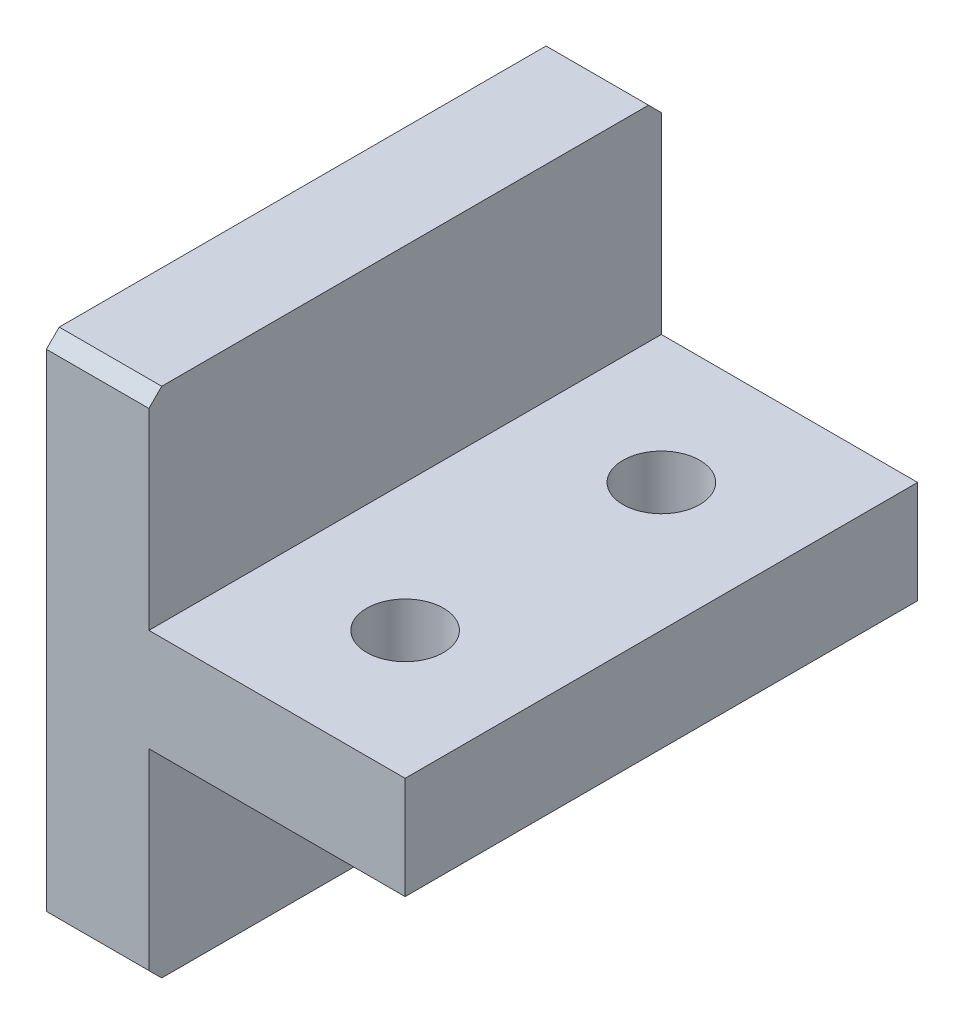
from build123d import *

# Parameters (mm, degrees)
SKETCH1_W               = 8
SKETCH1_H               = 40
BOSS_EXTRUDE1_DEPTH     = 40
CHAMFER1_SIZE           = 1
SKETCH2_W               = 20
SKETCH2_H               = 8
BOSS_EXTRUDE2_DEPTH     = 40
CUT_EXTRUDE1_DEPTH      = 55.405882035
CUT_EXTRUDE1_DEPTH_BACK = 55.405882035
SKETCH4_R               = 3


with BuildPart() as part:
    # Sketch1 → Boss-Extrude1 (new body)
    with BuildSketch(Plane(origin=(0, 0, 0), x_dir=(1, 0, 0), z_dir=(0, 1, 0))):
        with Locations((4, -20)):
            Rectangle(SKETCH1_W, SKETCH1_H)
    extrude(amount=BOSS_EXTRUDE1_DEPTH)

    # Chamfer1
    chamfer1_edges = [part.edges().sort_by_distance(p)[0] for p in [
        (4, 40, 0),
        (4, 0, 0),
        (4, 0, 40),
        (4, 40, 40),
    ]]
    chamfer(chamfer1_edges, length=CHAMFER1_SIZE)

    # Sketch2 → Boss-Extrude2 (add)
    with BuildSketch(Plane.XY.offset(40)):
        with Locations((18, 20)):
            Rectangle(SKETCH2_W, SKETCH2_H)
    extrude(amount=-BOSS_EXTRUDE2_DEPTH)

    # Sketch4 → Cut-Extrude1 (cut, two sides: drawn at the far end of the back side and taken through both)
    with BuildSketch(Plane(origin=(0, 24, 0), x_dir=(1, 0, 0), z_dir=(0, 1, 0)).offset(-CUT_EXTRUDE1_DEPTH_BACK)):
        with Locations(Location((18, -30, 0), (0, 0, 180))):
            Circle(SKETCH4_R)
        with Locations(Location((18, -10, 0), (0, 0, 180))):
            Circle(SKETCH4_R)
    extrude(amount=CUT_EXTRUDE1_DEPTH + CUT_EXTRUDE1_DEPTH_BACK, mode=Mode.SUBTRACT)


solid = part.part
